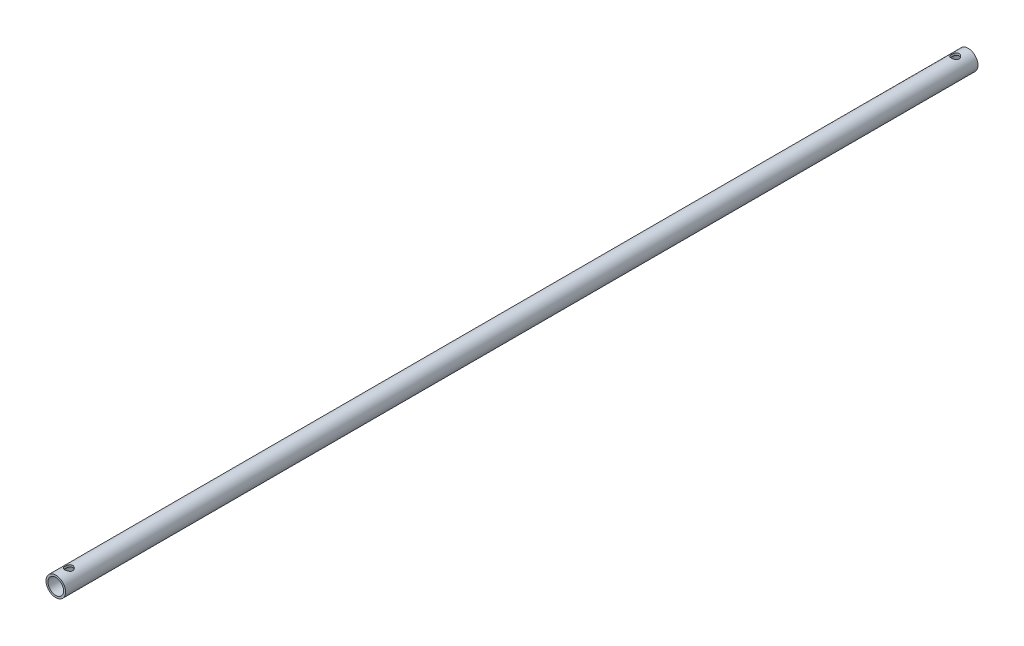
SolidWorks part; units mm, degrees
ref_plane "Front Plane" through (0, 0, 0) normal (0, 0, 1) x (1, 0, 0)
ref_plane "Top Plane" through (0, 0, 0) normal (0, 1, 0) x (1, 0, 0)
ref_plane "Right Plane" through (0, 0, 0) normal (1, 0, 0) x (0, 0, -1)
sketch "Sketch1" plane through (0, 0, 0) normal (0, 0, 1) x (1, 0, 0)
  circle A0 centre (0, 0) radius 7.5
  circle A1 centre (0, 0) radius 6
  dimension "D1" = 15
  dimension "D2" = 1.5
extrude "Boss-Extrude1" add sketch "Sketch1" along normal blind 700
sketch "Sketch2" plane through (0, 0, 0) normal (0, 1, 0) x (1, 0, 0)
  line L0 (0, -700) -> (0, 0) construction
  line L1 (-7.5, -700) -> (7.5, -700) construction
  line L4 (7.5, 0) -> (-7.5, 0) construction
  circle A0 centre (0, -10) radius 3
  circle A1 centre (0, -690) radius 3
  dimension "D1" = 6
  dimension "D2" = 10
  dimension "D3" = 6
  dimension "D4" = 10
extrude "Cut-Extrude1" cut sketch "Sketch2" against normal through all both and the other way through all
